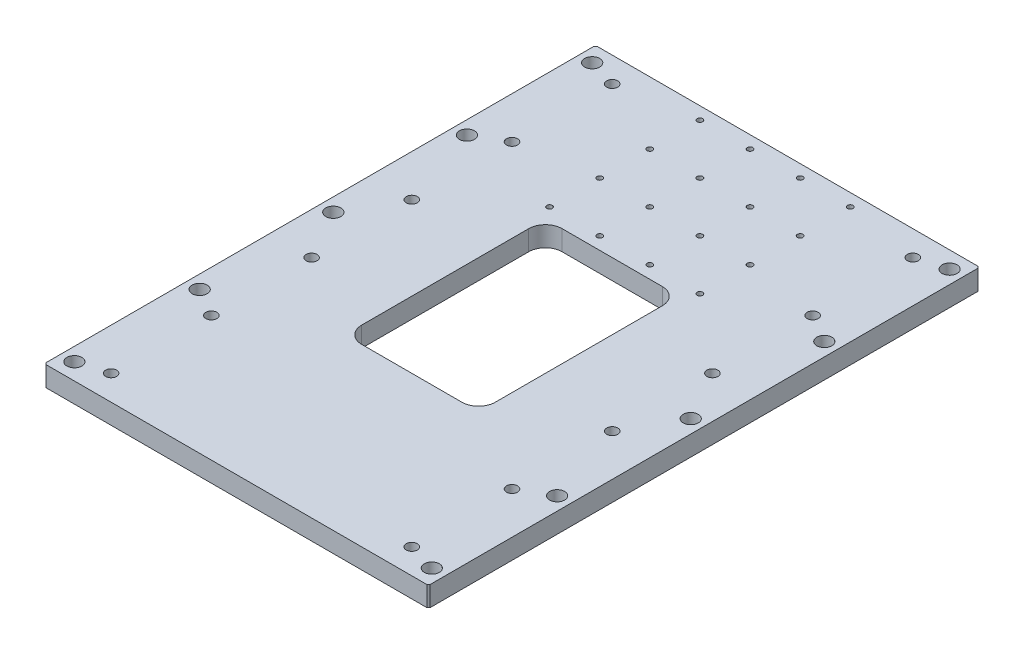
SolidWorks part; units mm, degrees
material "A6061"
ref_plane "前基準面" through (0, 0, 0) normal (0, 0, 1) x (1, 0, 0)
ref_plane "上基準面" through (0, 0, 0) normal (0, 1, 0) x (1, 0, 0)
ref_plane "右基準面" through (0, 0, 0) normal (1, 0, 0) x (0, 0, -1)
sketch "草图1" plane through (0, 0, 0) normal (0, 1, 0) x (1, 0, 0)
  line L1 (-115, -165) -> (115, -165)
  line L2 (-115, -165) -> (-115, 165)
  line L3 (-115, 165) -> (115, 165)
  line L4 (115, -165) -> (115, 165)
  line L5 (-115, -165) -> (115, 165) construction
  line L6 (-115, 165) -> (115, -165) construction
  point P0 (0, 0)
  dimension "D1" = 230
  dimension "D2" = 330
extrude "凸台-拉伸1" add sketch "草图1" along normal mid plane 12
hole_wizard "M8 间隙孔1" positions "草图3" profile "草图2" hole size "M8" standard "GB" end condition through all
sketch "草图3" plane through (0, 6, 0) normal (0, 1, 0) x (1, 0, 0)
  line L0 (0, 179.242) -> (0, 0) construction
  line L1 (0, 0) -> (-127.5616, 0) construction
  point P0 (-107, 155)
  point P2 (-107, 80)
  point P17 (107, 80)
  point P18 (107, 155)
  point P28 (-107, 0)
  point P31 (-107, -155)
  point P32 (-107, -80)
  point P34 (107, -80)
  point P35 (107, -155)
  point P37 (107, 0)
  dimension "D1" = 214
  dimension "D2" = 75
  dimension "D3" = 80
sketch "草图2" plane through (-107, 6, -155) normal (1, 0, 0) x (0, 0, 1)
  line L0 (0, 0) -> (0, 12)
  line L1 (0, 12) -> (4.5, 12)
  line L2 (4.5, 12) -> (4.5, 0)
  line L5 (4.5, 0) -> (0, 0)
  line L11 (0, -6.35) -> (0, 107.95) construction
  dimension "通孔孔直径" = 9
  dimension "通孔孔深度" = 12
chamfer "倒角1" distance 1 angle 45 4 edges at (115, 0, 165) (-115, 0, 165) (115, 0, -165) (-115, 0, -165)
hole_wizard "打孔尺寸(%根据)内六角圆柱头螺钉的类型1" positions "草图5" profile "草图4" counterbore size "M6" standard "GB" end condition through all
sketch "草图5" plane through (0, -6, 0) normal (0, -1, 0) x (-1, 0, 0)
  line L0 (0, -268.7796) -> (0, 0) construction
  line L1 (0, 0) -> (119.8163, 0) construction
  point P0 (90, -150)
  point P16 (-90, -150)
  point P28 (90, -90)
  point P29 (-90, -90)
  point P30 (90, -30)
  point P31 (-90, -30)
  point P32 (90, 30)
  point P33 (-90, 30)
  point P34 (90, 90)
  point P35 (-90, 90)
  point P36 (90, 150)
  point P37 (-90, 150)
  dimension "D1" = 6
  dimension "D2" = 60
  dimension "D3" = 180
sketch "草图4" plane through (-90, -6, 150) normal (1, 0, 0) x (0, 0, -1)
  line L0 (0, 0) -> (0, 12)
  line L1 (0, 12) -> (3.3, 12)
  line L3 (3.3, 12) -> (3.3, 6.8)
  line L4 (3.3, 6.8) -> (5.5, 6.8)
  line L5 (5.5, 6.8) -> (5.5, 0)
  line L7 (5.5, 0) -> (0, 0)
  line L11 (0, -6.35) -> (0, 107.95) construction
  dimension "通孔孔直径" = 6.6
  dimension "通孔孔深度" = 12
  dimension "柱形沉头孔直径" = 11
  dimension "柱形沉头孔深度" = 6.8
sketch "草图6" plane through (0, 6, 0) normal (0, 1, 0) x (1, 0, 0)
  line L1 (-40, -60) -> (40, -60)
  line L2 (-40, -60) -> (-40, 60)
  line L3 (-40, 60) -> (40, 60)
  line L4 (40, -60) -> (40, 60)
  line L5 (-40, -60) -> (40, 60) construction
  line L6 (-40, 60) -> (40, -60) construction
  point P0 (0, 0)
  dimension "D1" = 120
  dimension "D2" = 80
extrude "切除-拉伸1" cut sketch "草图6" against normal through all
fillet "圆角1" radius 10 4 edges at (40, 0, 60) (-40, 0, 60) (-40, 0, -60) (40, 0, -60)
hole_wizard "M4 螺纹孔1" positions "草图10" profile "草图9" tap size "M4" standard "GB" end condition through all
sketch "草图10" plane through (0, 6, 0) normal (0, 1, 0) x (1, 0, 0)
  line L0 (0, 165) -> (0, 60) construction
  line L1 (114, 165) -> (-114, 165) construction
  line L2 (30, 60) -> (-30, 60) construction
  line L4 (0, 112.5) -> (-131.3886, 112.5) construction
  point P30 (-45, 157.5)
  point P51 (-15, 157.5)
  point P52 (15, 157.5)
  point P53 (45, 157.5)
  point P54 (-15, 127.5)
  point P55 (15, 127.5)
  point P56 (45, 127.5)
  point P57 (-15, 97.5)
  point P58 (15, 97.5)
  point P59 (45, 97.5)
  point P60 (-15, 67.5)
  point P61 (15, 67.5)
  point P62 (45, 67.5)
  point P63 (-45, 127.5)
  point P64 (-45, 97.5)
  point P65 (-45, 67.5)
  dimension "D1" = 4
  dimension "D2" = 4
  dimension "D3" = 30
  dimension "D4" = 30
sketch "草图9" plane through (-45, 6, -67.5) normal (1, 0, 0) x (0, 0, 1)
  line L0 (0, 0) -> (0, 12)
  line L1 (0, 12) -> (1.65, 12)
  line L2 (1.65, 12) -> (1.65, 0)
  line L5 (1.65, 0) -> (0, 0)
  line L11 (0, -6.35) -> (0, 107.95) construction
  dimension "通孔螺纹孔钻头直径" = 3.3
  dimension "通孔螺纹孔钻头深度" = 12
cosmetic thread "孔螺蚊线3" parameters "D2"=4
cosmetic thread "孔螺蚊线4" parameters "D2"=4
cosmetic thread "孔螺蚊线5" parameters "D2"=4
cosmetic thread "孔螺蚊线6" parameters "D2"=4
cosmetic thread "孔螺蚊线7" parameters "D2"=4
cosmetic thread "孔螺蚊线8" parameters "D2"=4
cosmetic thread "孔螺蚊线9" parameters "D2"=4
cosmetic thread "孔螺蚊线10" parameters "D2"=4
cosmetic thread "孔螺蚊线11" parameters "D2"=4
cosmetic thread "孔螺蚊线12" parameters "D2"=4
cosmetic thread "孔螺蚊线13" parameters "D2"=4
cosmetic thread "孔螺蚊线14" parameters "D2"=4
cosmetic thread "孔螺蚊线15" parameters "D2"=4
cosmetic thread "孔螺蚊线16" parameters "D2"=4
cosmetic thread "孔螺蚊线17" parameters "D2"=4
cosmetic thread "孔螺蚊线18" parameters "D2"=4
